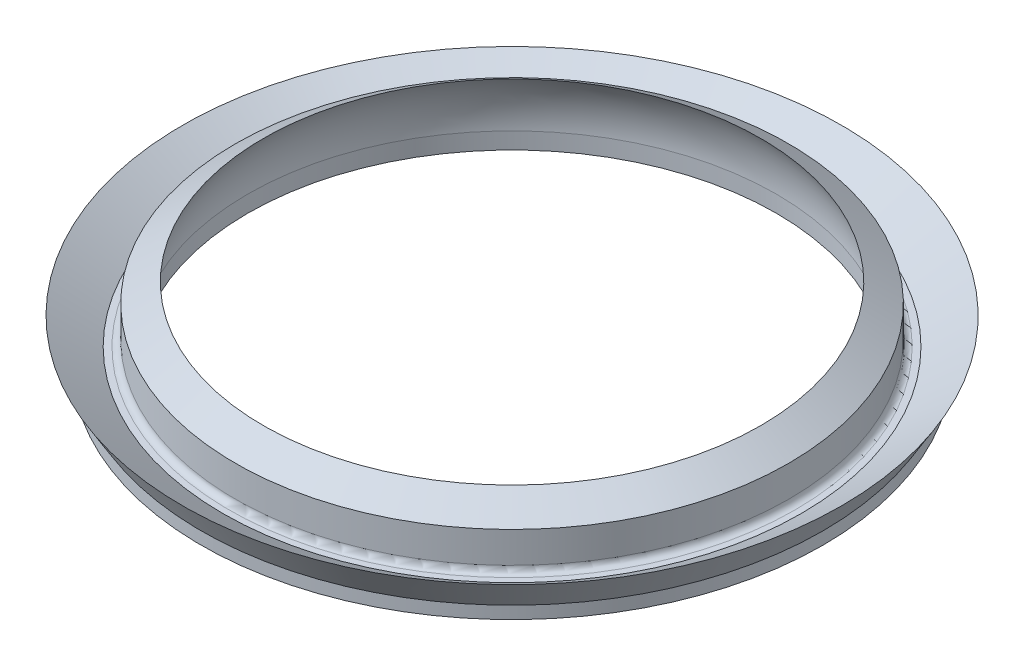
from build123d import *


with BuildPart() as part:
    # 草图1 → 旋转1 (revolve)
    with BuildSketch(Plane.XY):
        with BuildLine():
            Line((42.5, -6.169872981), (49.995512501, -6.169872981))
            Line((49.995512501, -6.169872981), (49.995512501, -4.169872981))
            Line((49.995512501, -4.169872981), (53, 0.830127019))
            Line((53, 0.830127019), (46.5, -3.5))
            Line((46.5, -3.5), (45.5, -3.5))
            ThreePointArc((45.5, -3.5), (44.792893219, -3.207106781), (44.5, -2.5))
            Line((44.5, -2.5), (44.5, 2.5))
            Line((44.5, 2.5), (40, 5.5))
            ThreePointArc((40, 5.5), (41.968412898, 1.199559138), (42.5, -3.5))
            Line((42.5, -3.5), (42.5, -6.169872981))
        make_face()
    revolve(axis=Axis((0, -5.5, 0), (0, 1, 0)))


solid = part.part
